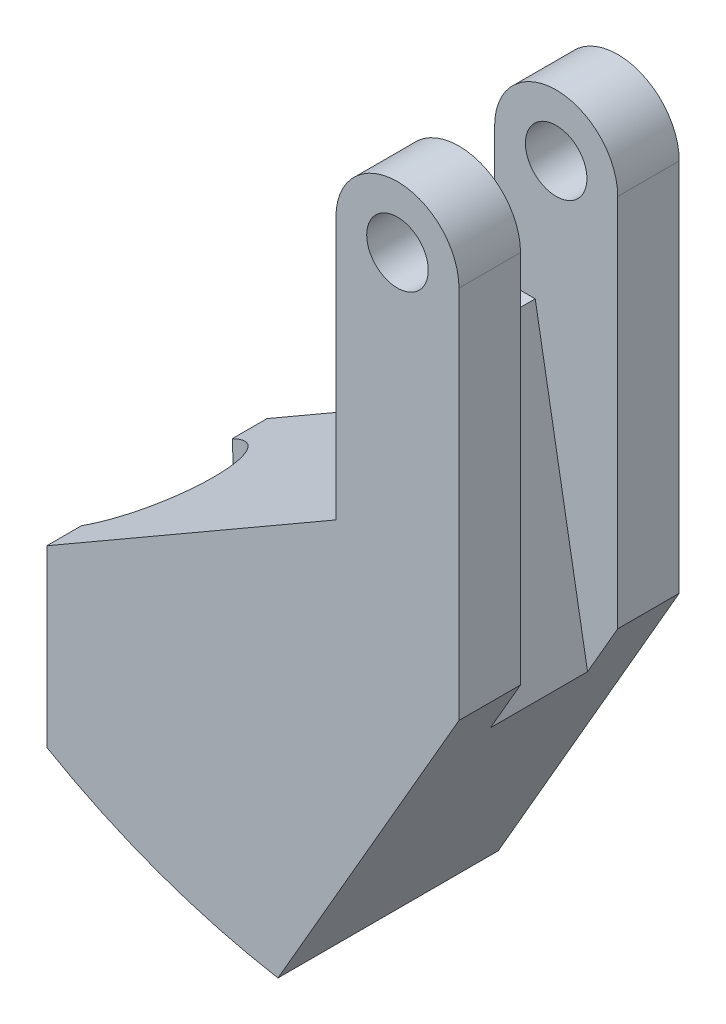
SolidWorks part; units mm, degrees
ref_plane "Front Plane" through (0, 0, 0) normal (0, 0, 1) x (1, 0, 0)
ref_plane "Top Plane" through (0, 0, 0) normal (0, 1, 0) x (1, 0, 0)
ref_plane "Right Plane" through (0, 0, 0) normal (1, 0, 0) x (0, 0, -1)
sketch "Sketch2" plane through (0, 0, 0) normal (0, 0, 1) x (1, 0, 0)
  line L0 (5, -30.431) -> (5, 0)
  line L1 (-5, 0) -> (-5, -21.3161)
  line L2 (-5, -21.3161) -> (-28.5, -34.8838)
  line L3 (-28.5, -34.8838) -> (-28.5, -49.0746)
  line L4 (-9.7119, -55.9128) -> (5, -30.431)
  arc A0 (5, 0) -> (-5, 0) centre (0, 0) ccw
  arc A1 (-28.5, -49.0746) -> (-9.7119, -55.9128) centre (0, 0) ccw
  circle A2 centre (0, 0) radius 2.5
  dimension "D1" = 2.5
extrude "Boss-Extrude1" add sketch "Sketch2" along normal blind 17.9
ref_plane "Plane2" through (0, 0, 8.95) normal (0, 0, -1) x (-1, 0, 0)
sketch "Sketch3" plane through (0, 0, 8.95) normal (0, 0, -1) x (-1, 0, 0)
  line L0 (1.8486, -9.7288) -> (5, -10.2844) construction
  line L1 (5, 0) -> (5, -21.3161) construction
  line L2 (5, -21.3161) -> (28.5, -34.8838) construction
  line L3 (1.8486, -9.7288) -> (-2.55, -34.6745)
  line L4 (9.7119, -55.9128) -> (-5, -30.431) construction
  line L5 (-2.55, -34.6745) -> (-5, -30.431)
  line L6 (-5, -30.431) -> (-5, -8.5212)
  line L7 (-5, -30.431) -> (-5, 0) construction
  line L8 (1.8486, -9.7288) -> (-5, -8.5212)
  dimension "D1" = 160
  dimension "D2" = 3.2
  dimension "D3" = 90
  dimension "D4" = 4.9
extrude "Cut-Extrude1" cut sketch "Sketch3" against normal mid plane 7.9
sketch "Sketch4" plane through (-5, 0, 0) normal (-1, 0, 0) x (0, 0, 1)
  line L6 (8.95, 0) -> (8.95, 10.7149) construction
  line L7 (17.9, 0) -> (0, 0) construction
  line L8 (8.95, 18.425) -> (8.95, -18.425) construction
  line L9 (5, -10.5561) -> (5, 7.3299)
  line L10 (5, 7.3299) -> (12.9, 7.3299)
  line L11 (12.9, 7.3299) -> (12.9, -10.5561)
  line L12 (5, -10.5561) -> (12.9, -10.5561)
  dimension "D2" = 7.9
extrude "Cut-Extrude2" cut sketch "Sketch4" against normal blind 41.9
ref_plane "Plane3" through (19.4096, -53.3276, 0) normal (0.342, -0.9397, 0) x (0, 0, -1)
sketch "Sketch5" plane through (19.4096, -53.3276, 0) normal (0.342, -0.9397, 0) x (0, 0, -1)
  line L0 (-17.9, -28.2495) -> (0, -28.2495) construction
  circle A0 centre (-8.95, -39.6677) radius 6.2
  point P5 (-8.95, -28.2495)
  dimension "D1" = 12.4
extrude "Cut-Extrude3" cut sketch "Sketch5" against normal blind 41.9
